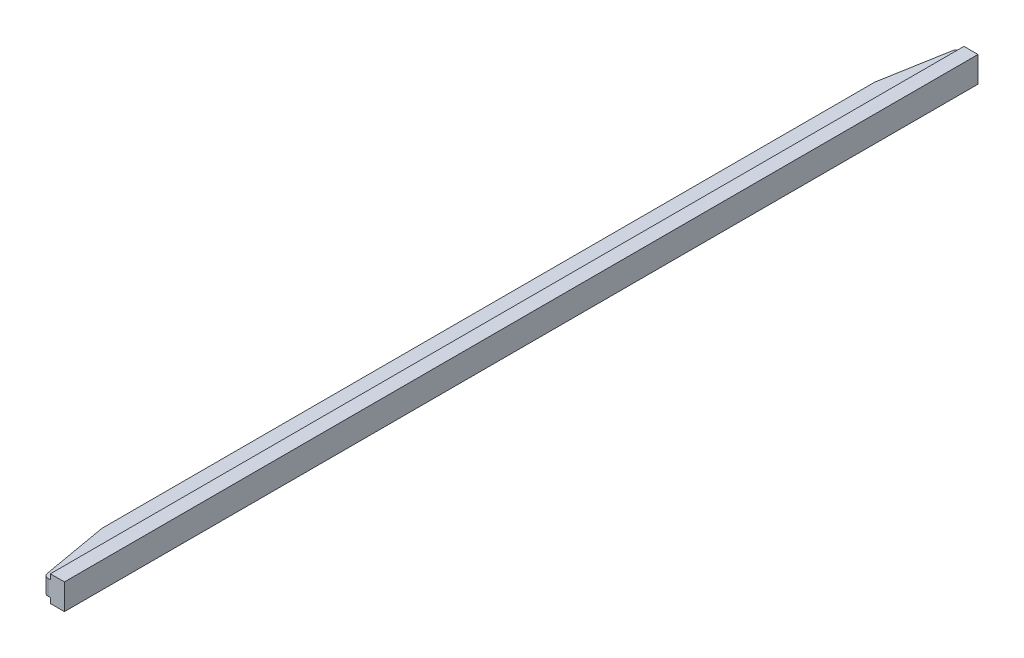
SolidWorks part; units mm, degrees
material "Nylon 101"
ref_plane "Front" through (0, 0, 0) normal (0, 0, 1) x (1, 0, 0)
ref_plane "Top" through (0, 0, 0) normal (0, 1, 0) x (1, 0, 0)
ref_plane "Right" through (0, 0, 0) normal (1, 0, 0) x (0, 0, -1)
sketch "Sketch1" plane through (0, 0, 0) normal (0, 0, 1) x (1, 0, 0)
  line L0 (0, -5.5) -> (0, 5.5)
  line L1 (0, 5.5) -> (-6, 5.5)
  line L2 (-6, 5.5) -> (-6, 3.3)
  line L3 (-6, 3.3) -> (-14, 3.3)
  line L4 (-14, 3.3) -> (-14, -3.3)
  line L5 (-14, 0) -> (0, 0) construction
  line L6 (-6, -3.3) -> (-14, -3.3)
  line L7 (-6, -5.5) -> (-6, -3.3)
  line L8 (0, -5.5) -> (-6, -5.5)
  dimension "D1" = 14
  dimension "D2" = 6
  dimension "D3" = 11
  dimension "D4" = 6.6
extrude "Boss-Extrude1" add sketch "Sketch1" along normal mid plane 390
chamfer "Chamfer1" distance 30 angle 10 2 edges at (-14, 0, -195) (-14, 0, 195)
fillet "Fillet1" radius 2 4 edges at (-8.7102, 0, 195) (-14, 0, 165) (-14, 0, -165) (-8.7102, 0, -195)
